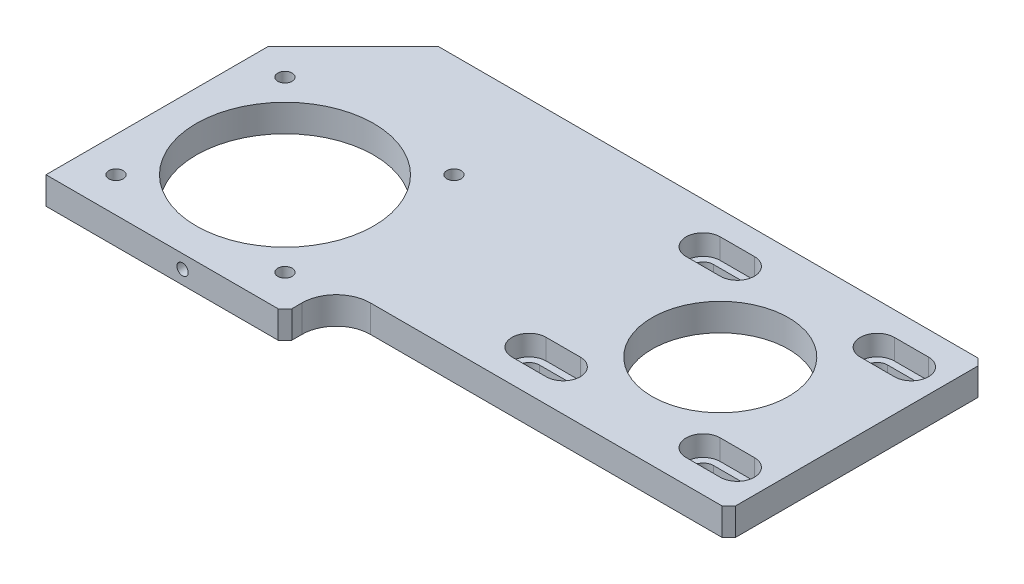
SolidWorks part; units mm, degrees
ref_plane "前视基准面" through (0, 0, 0) normal (0, 0, 1) x (1, 0, 0)
ref_plane "上视基准面" through (0, 0, 0) normal (0, 1, 0) x (1, 0, 0)
ref_plane "右视基准面" through (0, 0, 0) normal (1, 0, 0) x (0, 0, -1)
sketch "草图2" plane through (0, 0, 0) normal (0, 1, 0) x (1, 0, 0)
  line L1 (-92.5, 45) -> (92.5, 45)
  line L2 (-92.5, 45) -> (-92.5, -45)
  line L3 (-92.5, -45) -> (92.5, -45)
  line L4 (92.5, 45) -> (92.5, -45)
  line L5 (-92.5, 45) -> (92.5, -45) construction
  line L6 (-92.5, -45) -> (92.5, 45) construction
  point P0 (0, 0)
  dimension "D1" = 185
  dimension "D2" = 90
extrude "凸台-拉伸1" add sketch "草图2" along normal blind 8
sketch "草图4" plane through (0, 8, 0) normal (0, 1, 0) x (1, 0, 0)
  line L0 (-92.5, 45) -> (-92.5, -45) construction
  line L1 (92.5, -45) -> (-22.5, -45)
  line L2 (92.5, -45) -> (92.5, -30)
  line L3 (92.5, -30) -> (-22.5, -30)
  line L4 (-22.5, -45) -> (-22.5, -30)
  dimension "D1" = 70
  dimension "D2" = 15
extrude "切除-拉伸7" cut sketch "草图4" against normal through all
sketch "草图5" plane through (0, 8, 0) normal (0, 1, 0) x (1, 0, 0)
  line L0 (92.5, 45) -> (-92.5, 45) construction
  line L1 (-92.5, 45) -> (-92.5, -45) construction
  circle A0 centre (-57.5, -10) radius 26
  dimension "D1" = 52
  dimension "D2" = 55
  dimension "D3" = 35
extrude "切除-拉伸8" cut sketch "草图5" against normal through all
hole_wizard "M5 螺纹孔1" positions "草图9" profile "草图8" tap size "M5" standard "ISO" end condition through all
sketch "草图9" plane through (0, 8, 0) normal (0, 1, 0) x (1, 0, 0)
  line L0 (-57.5, -10) -> (-82.2487, 14.7487) construction
  line L2 (-57.5, -10) -> (-32.7513, 14.7487) construction
  line L4 (-57.5, -10) -> (-57.5, 43.1497)
  circle A0 centre (-57.5, -10) radius 35 construction
  point P23 (-82.2487, 14.7487)
  point P38 (-32.7513, 14.7487)
  point P39 (-32.7513, -34.7487)
  point P40 (-82.2487, -34.7487)
  point P41 (-57.5, -10)
  dimension "D1" = 70
  dimension "D2" = 90
  dimension "D3" = 45
  dimension "D4" = 4
sketch "草图8" plane through (-82.2487, 8, -14.7487) normal (1, 0, 0) x (0, 0, 1)
  line L0 (0, 0) -> (0, 8)
  line L1 (0, 8) -> (2.1, 8)
  line L2 (2.1, 8) -> (2.1, 0)
  line L5 (2.1, 0) -> (0, 0)
  line L11 (0, -6.35) -> (0, 107.95) construction
  dimension "通孔螺纹孔钻头直径" = 4.2
  dimension "通孔螺纹孔钻头深度" = 8
cosmetic thread "孔螺蚊线1" parameters "D2"=5
cosmetic thread "孔螺蚊线2" parameters "D2"=5
cosmetic thread "孔螺蚊线3" parameters "D2"=5
cosmetic thread "孔螺蚊线4" parameters "D2"=5
sketch "草图10" plane through (0, 8, 0) normal (0, 1, 0) x (1, 0, 0)
  line L0 (92.5, -30) -> (92.5, 45) construction
  line L1 (92.5, 45) -> (-92.5, 45) construction
  circle A0 centre (52.5, 7.5) radius 20
  dimension "D1" = 40
  dimension "D2" = 40
  dimension "D3" = 37.5
extrude "切除-拉伸9" cut sketch "草图10" against normal through all
sketch "草图15" plane through (0, 8, 0) normal (0, 1, 0) x (1, 0, 0)
  line L0 (95.3933, 7.5) -> (-6.8668, 7.5) construction
  line L1 (73, -18) -> (83, -18) construction
  line L2 (73, -13) -> (83, -13)
  line L3 (73, -23) -> (83, -23)
  line L4 (92.5, -30) -> (92.5, 45) construction
  line L5 (73, 33) -> (83, 33) construction
  line L6 (73, 28) -> (83, 28)
  line L7 (73, 38) -> (83, 38)
  line L8 (22, -18) -> (32, -18) construction
  line L9 (22, -13) -> (32, -13)
  line L10 (22, -23) -> (32, -23)
  line L11 (22, 33) -> (32, 33) construction
  line L12 (22, 28) -> (32, 28)
  line L13 (22, 38) -> (32, 38)
  arc A0 (73, -13) -> (73, -23) centre (73, -18) ccw
  arc A1 (83, -23) -> (83, -13) centre (83, -18) ccw
  arc A2 (73, 28) -> (73, 38) centre (73, 33) cw
  arc A3 (83, 38) -> (83, 28) centre (83, 33) cw
  arc A4 (22, -13) -> (22, -23) centre (22, -18) ccw
  arc A5 (32, -23) -> (32, -13) centre (32, -18) ccw
  arc A6 (22, 28) -> (22, 38) centre (22, 33) cw
  arc A7 (32, 38) -> (32, 28) centre (32, 33) cw
  point P5 (78, -18)
  point P14 (78, 33)
  point P23 (27, -18)
  point P30 (27, 33)
  dimension "D3" = 9.5
  dimension "D4" = 51
  dimension "D1" = 10
  dimension "D2" = 10
  dimension "D5" = 2
extrude "切除-拉伸15" cut sketch "草图15" against normal blind 6
sketch "草图16" plane through (0, 2, 0) normal (0, 1, 0) x (1, 0, 0)
  line L0 (73, -18) -> (83, -18) construction
  line L1 (73, -15) -> (83, -15)
  line L2 (73, -21) -> (83, -21)
  line L4 (97.6204, 7.5) -> (10.9498, 7.5) construction
  line L5 (73, 33) -> (83, 33) construction
  line L6 (73, 30) -> (83, 30)
  line L7 (73, 36) -> (83, 36)
  line L8 (22, -18) -> (32, -18) construction
  line L9 (22, -15) -> (32, -15)
  line L10 (22, -21) -> (32, -21)
  line L11 (22, 33) -> (32, 33) construction
  line L12 (22, 30) -> (32, 30)
  line L13 (22, 36) -> (32, 36)
  arc A0 (73, -15) -> (73, -21) centre (73, -18) ccw
  arc A1 (83, -21) -> (83, -15) centre (83, -18) ccw
  arc A2 (73, 30) -> (73, 36) centre (73, 33) cw
  arc A3 (83, 36) -> (83, 30) centre (83, 33) cw
  arc A4 (22, -15) -> (22, -21) centre (22, -18) ccw
  arc A5 (32, -21) -> (32, -15) centre (32, -18) ccw
  arc A6 (22, 30) -> (22, 36) centre (22, 33) cw
  arc A7 (32, 36) -> (32, 30) centre (32, 33) cw
  point P3 (78, -18)
  point P13 (78, 33)
  point P22 (27, -18)
  point P29 (27, 33)
  dimension "D3" = 2
  dimension "D1" = 10
  dimension "D2" = 6
extrude "切除-拉伸16" cut sketch "草图16" against normal through all
hole_wizard "M4 螺纹孔1" positions "草图18" profile "草图17" tap size "M4" standard "ISO"
sketch "草图18" plane through (0, 0, -45) normal (0, 0, -1) x (-1, 0, 0)
  line L0 (-92.5, 8) -> (92.5, 8) construction
  line L1 (-92.5, 8) -> (-92.5, 0) construction
  point P0 (-52.5, 4)
  point P2 (52.5, 4)
  dimension "D1" = 4
  dimension "D2" = 40
  dimension "D3" = 105
sketch "草图17" plane through (52.5, 4, -45) normal (1, 0, 0) x (0, 1, 0)
  line L0 (0, 0) -> (0, 12.9914)
  line L1 (0, 12.9914) -> (1.65, 12)
  line L2 (1.65, 12) -> (1.65, 0)
  line L5 (1.65, 0) -> (0, 0)
  line L10 (0, 12.9914) -> (-1.65, 12) construction
  line L11 (0, -6.35) -> (0, 107.95) construction
  dimension "螺纹孔钻头直径" = 3.3
  dimension "螺纹孔钻头深度" = 12
  dimension "导头角度" = 118
cosmetic thread "孔螺蚊线5" parameters "D1"=8, "D2"=4
cosmetic thread "孔螺蚊线6" parameters "D1"=8, "D2"=4
hole_wizard "M4 螺纹孔2" positions "草图20" profile "草图19" tap size "M4" standard "ISO"
sketch "草图20" plane through (0, 0, 45) normal (0, 0, 1) x (1, 0, 0)
  line L0 (-92.5, 8) -> (-22.5, 8) construction
  line L1 (92.5, 0) -> (92.5, 8) construction
  point P0 (-52.5, 4)
  dimension "D1" = 4
  dimension "D2" = 145
sketch "草图19" plane through (-52.5, 4, 45) normal (1, 0, 0) x (0, -1, 0)
  line L0 (0, 0) -> (0, 12.9914)
  line L1 (0, 12.9914) -> (1.65, 12)
  line L2 (1.65, 12) -> (1.65, 0)
  line L5 (1.65, 0) -> (0, 0)
  line L10 (0, 12.9914) -> (-1.65, 12) construction
  line L11 (0, -6.35) -> (0, 107.95) construction
  dimension "螺纹孔钻头直径" = 3.3
  dimension "螺纹孔钻头深度" = 12
  dimension "导头角度" = 118
cosmetic thread "孔螺蚊线7" parameters "D1"=8, "D2"=4
chamfer "倒角1" distance 25 angle 45 1 edges at (-92.5, 4, -45)
chamfer "倒角2" distance 2 angle 45 3 edges at (92.5, 4, -45) (92.5, 4, 30) (-22.5, 4, 45)
fillet "圆角1" radius 10 1 edges at (-22.5, 4, 30)
